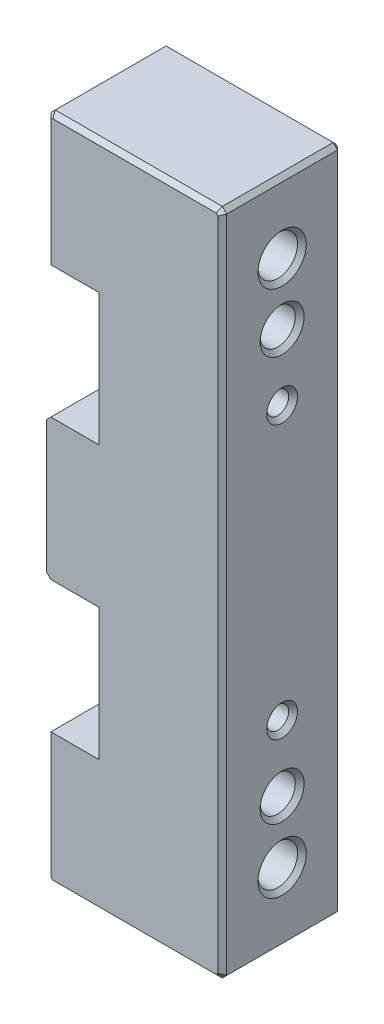
SolidWorks part; units mm, degrees
material "AL6061"
ref_plane "前视基准面" through (0, 0, 0) normal (0, 0, 1) x (1, 0, 0)
ref_plane "上视基准面" through (0, 0, 0) normal (0, 1, 0) x (1, 0, 0)
ref_plane "右视基准面" through (0, 0, 0) normal (1, 0, 0) x (0, 0, -1)
sketch "草图3" plane through (0, 0, 0) normal (0, 0, 1) x (1, 0, 0)
  line L0 (10, 37.5) -> (9.5, 38)
  line L1 (9.5, 38) -> (-9.5, 38)
  line L2 (-9.5, 38) -> (-10, 37.5)
  line L3 (-10, 37.5) -> (-10, 23.5)
  line L4 (-10, 23.5) -> (-9.5, 23)
  line L5 (-9.5, 23) -> (-2, 23)
  line L6 (-2, 23) -> (-2, 8)
  line L7 (-2, 8) -> (-9.5, 8)
  line L8 (-9.5, 8) -> (-10, 7.5)
  line L9 (-10, 7.5) -> (-10, -7.5)
  line L10 (-10, -7.5) -> (-9.5, -8)
  line L13 (-9.5, -8) -> (-2, -8)
  line L15 (-2, -8) -> (-2, -23)
  line L16 (-2, -23) -> (-9.5, -23)
  line L17 (-9.5, -23) -> (-10, -23.5)
  line L18 (-10, -23.5) -> (-10, -37.5)
  line L19 (-10, -37.5) -> (-9.5, -38)
  line L20 (-9.5, -38) -> (9.5, -38)
  line L22 (9.5, -38) -> (10, -37.5)
  line L23 (10, -37.5) -> (10, 37.5)
extrude "凸台-拉伸1" add sketch "草图3" against normal up to surface (13.6 mm away)
chamfer "倒角1" distance 0.5 angle 45 18 edges at (-10, 30.5, -13.6) (-9.75, 37.75, -13.6) (0, 38, -13.6) (9.75, 37.75, -13.6) (10, 0, -13.6) (9.75, -37.75, -13.6) (-10, -30.5, -13.6) (-9.75, -37.75, -13.6) (0, -38, -13.6) (-10, 30.5, 0) (-9.75, 37.75, 0) (0, 38, 0) (9.75, 37.75, 0) (10, 0, 0) (9.75, -37.75, 0) (-10, -30.5, 0) (-9.75, -37.75, 0) (0, -38, 0)
hole_wizard "M4 六角凹头螺钉的柱形沉头孔1" positions "草图4" profile "草图5" counterbore size "M4" standard "ISO" end condition through all
sketch "草图4" plane through (-10, 0, 0) normal (-1, 0, 0) x (0, 0, 1)
  point P0 (-6.8, -30)
  point P4 (-6.8, 30)
sketch "草图5" plane through (-10, -30, -6.8) normal (0, 1, 0) x (0, 0, 1)
  line L0 (0, 0) -> (0, 20)
  line L1 (0, 20) -> (2.25, 20)
  line L3 (2.25, 20) -> (2.25, 4.4)
  line L4 (2.25, 4.4) -> (4, 4.4)
  line L5 (4, 4.4) -> (4, 0)
  line L7 (4, 0) -> (0, 0)
  line L11 (0, -6.35) -> (0, 107.95) construction
  dimension "通孔孔直径" = 4.5
  dimension "通孔孔深度" = 20
  dimension "柱形沉头孔直径" = 8
  dimension "柱形沉头孔深度" = 4.4
sketch "草图6" plane through (0, 0, 0) normal (0, 0, 1) x (1, 0, 0)
  line L0 (-9.5, 23) -> (-2, 23) construction
  line L1 (-4, -8) -> (-2, -8)
  line L2 (-4, -8) -> (-4, -23)
  line L3 (-4, -23) -> (-2, -23)
  line L4 (-2, -8) -> (-2, -23)
  line L5 (-2, 8) -> (-4, 8)
  line L6 (-2, 8) -> (-2, 23)
  line L7 (-2, 23) -> (-4, 23)
  line L8 (-4, 8) -> (-4, 23)
extrude "凸台-拉伸2" add sketch "草图6" against normal up to surface (13.6 mm away)
hole_wizard "M3 螺纹孔1" positions "草图7" profile "草图8" tap size "M3" standard "ISO" end condition through all
sketch "草图7" plane through (-4, 0, 0) normal (-1, 0, 0) x (0, 0, 1)
  point P0 (-6.8, -15.5)
  point P3 (-6.8, 15.5)
sketch "草图8" plane through (-4, -15.5, -6.8) normal (0, 1, 0) x (0, 0, 1)
  line L0 (0, 0) -> (0, 14)
  line L1 (0, 14) -> (1.25, 14)
  line L2 (1.25, 14) -> (1.25, 0)
  line L5 (1.25, 0) -> (0, 0)
  line L11 (0, -6.35) -> (0, 107.95) construction
  dimension "通孔螺纹孔钻头直径" = 2.5
  dimension "通孔螺纹孔钻头深度" = 14
cosmetic thread "孔螺蚊线1" parameters "D2"=3
cosmetic thread "孔螺蚊线2" parameters "D2"=3
hole_wizard "大小mm 暗销孔1" positions "草图9" profile "草图11" hole size "Ø4.0" standard "ISO"
sketch "草图9" plane through (10, 0, 0) normal (1, 0, 0) x (0, 0, -1)
  point P0 (6.8, -23)
  point P3 (6.8, 23)
sketch "草图11" plane through (10, -23, -6.8) normal (0, 1, 0) x (0, 0, -1)
  line L0 (0, 0) -> (0, 11.2017)
  line L1 (0, 11.2017) -> (2, 10)
  line L2 (2, 10) -> (2, 0)
  line L5 (2, 0) -> (0, 0)
  line L10 (0, 11.2017) -> (-2, 10) construction
  line L11 (0, -6.35) -> (0, 107.95) construction
  dimension "孔直径" = 4
  dimension "孔深度" = 10
  dimension "导头角度" = 118
chamfer "倒角2" distance 0.5 angle 45 8 edges at (-10, 30, -2.8) (-10, -30, -2.8) (10, -30, -4.55) (10, -23, -8.8) (10, -15.5, -5.55) (10, 15.5, -5.55) (10, 23, -8.8) (10, 30, -4.55)
hole_wizard "大小mm 暗销孔2" positions "草图13" profile "草图15" hole size "Ø3.0" standard "ISO"
sketch "草图13" plane through (-10, 0, 0) normal (-1, 0, 0) x (0, 0, 1)
  line L0 (-13.6, 0) -> (0, 0) construction
  line L1 (-13.6, 7.5) -> (-13.6, -7.5) construction
  point P0 (-6.8, 0)
sketch "草图15" plane through (-10, 0, -6.8) normal (0, 1, 0) x (0, 0, 1)
  line L0 (0, 0) -> (0, 1.9013)
  line L1 (0, 1.9013) -> (1.5, 1)
  line L2 (1.5, 1) -> (1.5, 0)
  line L5 (1.5, 0) -> (0, 0)
  line L10 (0, 1.9013) -> (-1.5, 1) construction
  line L11 (0, -6.35) -> (0, 107.95) construction
  dimension "孔直径" = 3
  dimension "孔深度" = 1
  dimension "导头角度" = 118
